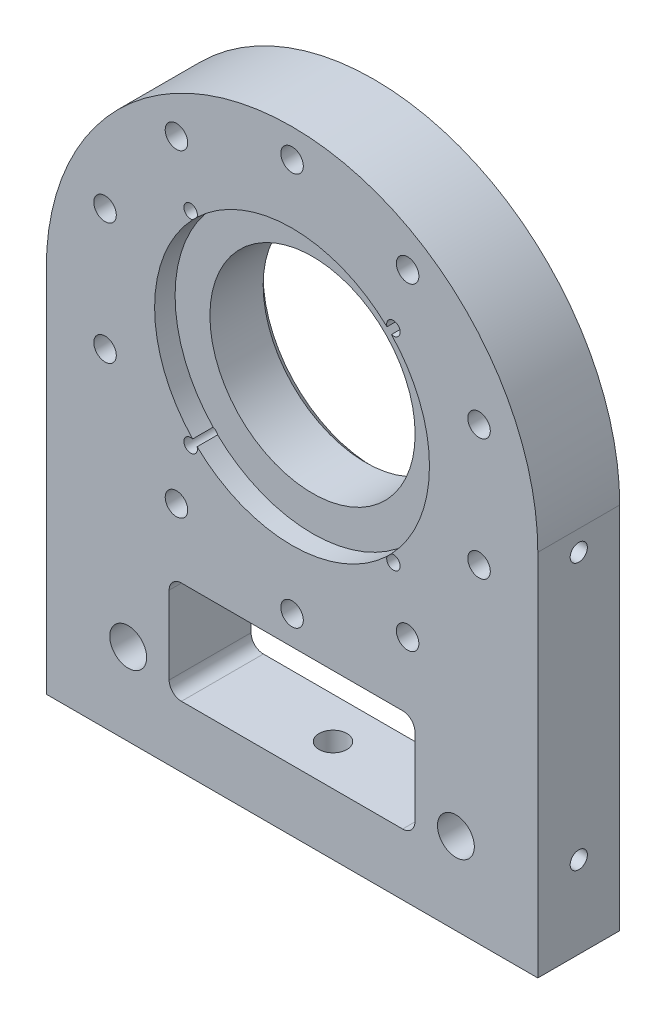
from build123d import *

# Parameters (mm, degrees)
SKETCH_1_R                  = 25.05
EXTRUDE_1_DEPTH             = 10
HOLE_WIZARD_M8_1_D          = 6.8
HOLE_WIZARD_M8_1_DEPTH      = 33.75
HOLE_WIZARD_M8_1_TIP        = 2.042926105
HOLE_WIZARD_6_0_6_1_D       = 6
HOLE_WIZARD_6_0_6_1_DEPTH   = 15
HOLE_WIZARD_6_0_6_1_TIP     = 1.802581857
SKETCH_6_R                  = 33.55
CUT_EXTRUDE_1_DEPTH         = 5
HOLE_WIZARD_M4_1_D          = 3.3
PATTERN_CIRCULAR_1_COUNT    = 4
CHAMFER_1_SIZE              = 2
HOLE_WIZARD_2_D             = 5.5
HOLE_WIZARD_2_CBORE_D       = 10
HOLE_WIZARD_2_CBORE_DEPTH   = 5.7
PATTERN_CIRCULAR_2_COUNT    = 10
HOLE_WIZARD_2_2_D           = 9
HOLE_WIZARD_2_2_CBORE_D     = 15
HOLE_WIZARD_2_2_CBORE_DEPTH = 9
CUT_EXTRUDE_2_DEPTH         = 163.788205961
HOLE_WIZARD_M5_1_AT_2_COUNT = 2
HOLE_WIZARD_M5_1_AT_2_PITCH = 65


with BuildPart() as part:
    # 草图1 → 凸台-拉伸1 (new, symmetric)
    with BuildSketch(Plane.XY):
        with BuildLine():
            Line((-60, 90), (-60, 0))
            Line((-60, 0), (60, 0))
            Line((60, 0), (60, 90))
            ThreePointArc((60, 90), (0, 150), (-60, 90))
        make_face()
        with Locations((0, 95)):
            Circle(SKETCH_1_R, mode=Mode.SUBTRACT)
    extrude(amount=EXTRUDE_1_DEPTH, both=True)

    # M8 螺纹孔1
    with Locations(Plane(origin=(0, 0, 0), x_dir=(-1, 0, 0), z_dir=(0, -1, 0))):
        with Locations((50, 0), (0, 0), (-50, 0)):
            Hole(HOLE_WIZARD_M8_1_D / 2, depth=HOLE_WIZARD_M8_1_DEPTH)
            with Locations((0, 0, -(HOLE_WIZARD_M8_1_DEPTH + HOLE_WIZARD_M8_1_TIP / 2))):  # 118° drill point
                Cone(0, HOLE_WIZARD_M8_1_D / 2, HOLE_WIZARD_M8_1_TIP, mode=Mode.SUBTRACT)

    # Ø6.0 (6) 直径孔1
    with Locations(Plane(origin=(0, 0, 0), x_dir=(-1, 0, 0), z_dir=(0, -1, 0))):
        with Locations((-35, 0), (35, 0)):
            Hole(HOLE_WIZARD_6_0_6_1_D / 2, depth=HOLE_WIZARD_6_0_6_1_DEPTH)
            with Locations((0, 0, -(HOLE_WIZARD_6_0_6_1_DEPTH + HOLE_WIZARD_6_0_6_1_TIP / 2))):  # 118° drill point
                Cone(0, HOLE_WIZARD_6_0_6_1_D / 2, HOLE_WIZARD_6_0_6_1_TIP, mode=Mode.SUBTRACT)

    # 草图6 → 切除-拉伸1 (cut)
    with BuildSketch(Plane.XY.offset(10)):
        with Locations((0, 95)):
            Circle(SKETCH_6_R)
    extrude(amount=-CUT_EXTRUDE_1_DEPTH, mode=Mode.SUBTRACT)

    # M4 螺纹孔1 (through all)
    with Locations(Plane(origin=(0, 0, -10), x_dir=(-1, 0, 0), z_dir=(0, 0, -1))):
        with Locations((-24.748737342, 119.748737342)):
            hole_wizard_m4_1 = Hole(HOLE_WIZARD_M4_1_D / 2)

    # 阵列(圆周)1: M4 螺纹孔1 ×4 about axis
    pattern_circular_1_axis = Axis((0, 95, 0), (0, 0, 1))
    for i in range(1, PATTERN_CIRCULAR_1_COUNT):
        add(hole_wizard_m4_1.rotate(pattern_circular_1_axis, i * 360 / PATTERN_CIRCULAR_1_COUNT), mode=Mode.SUBTRACT)

    # 倒角1
    chamfer_1_edges = [part.edges().sort_by_distance(p)[0] for p in [
        (-25.05, 95, -10),
    ]]
    chamfer(chamfer_1_edges, length=CHAMFER_1_SIZE)

    # Hole Wizard 2 (through all)
    with Locations(Plane(origin=(0, 0, -10), x_dir=(-1, 0, 0), z_dir=(0, 0, -1))):
        with Locations((0, 143)):
            hole_wizard_2 = CounterBoreHole(HOLE_WIZARD_2_D / 2, HOLE_WIZARD_2_CBORE_D / 2, HOLE_WIZARD_2_CBORE_DEPTH)

    # 阵列(圆周)2: Hole Wizard 2 ×10 about axis
    pattern_circular_2_axis = Axis((0, 95, 0), (0, 0, 1))
    for i in range(1, PATTERN_CIRCULAR_2_COUNT):
        add(hole_wizard_2.rotate(pattern_circular_2_axis, i * 360 / PATTERN_CIRCULAR_2_COUNT), mode=Mode.SUBTRACT)

    # Hole Wizard 2 2 (through all)
    with Locations(Plane(origin=(0, 0, -10), x_dir=(-1, 0, 0), z_dir=(0, 0, -1))):
        with Locations((-40, 20), (40, 20)):
            CounterBoreHole(HOLE_WIZARD_2_2_D / 2, HOLE_WIZARD_2_2_CBORE_D / 2, HOLE_WIZARD_2_2_CBORE_DEPTH)

    # 草图13 → 切除-拉伸2 (cut, through all)
    with BuildSketch(Plane(origin=(0, 0, -10), x_dir=(-1, 0, 0), z_dir=(0, 0, -1))):
        with BuildLine():
            Line((-27, 40), (27, 40))
            ThreePointArc((27, 40), (29.121320344, 39.121320344), (30, 37))
            Line((30, 37), (30, 18))
            ThreePointArc((30, 18), (29.121320344, 15.878679656), (27, 15))
            Line((27, 15), (-27, 15))
            ThreePointArc((-27, 15), (-29.121320344, 15.878679656), (-30, 18))
            Line((-30, 18), (-30, 37))
            ThreePointArc((-30, 37), (-29.121320344, 39.121320344), (-27, 40))
        make_face()
    extrude(amount=-CUT_EXTRUDE_2_DEPTH, mode=Mode.SUBTRACT)

    # 草图15 → M5 螺纹孔1 (revolve, cut)
    with BuildSketch(Plane(origin=(60, 20, 0), x_dir=(0, 0, -1), z_dir=(0, 1, 0))):
        Polygon((0, 0), (0, 15.6618073), (2.1, 14.4), (2.1, 0), align=None)
    hole_wizard_m5_1 = revolve(axis=Axis((66.35, 20, 0), (-1, 0, 0)), mode=Mode.SUBTRACT)

    # M5 螺纹孔1 at 2: M5 螺纹孔1 ×2
    with Locations(*[(0, i * HOLE_WIZARD_M5_1_AT_2_PITCH, 0) for i in range(1, HOLE_WIZARD_M5_1_AT_2_COUNT)]):
        add(hole_wizard_m5_1, mode=Mode.SUBTRACT)

    # 镜向1: M5 螺纹孔1 across plane
    add(hole_wizard_m5_1.mirror(Plane(origin=(0, 0, 0), x_dir=(0, 0, 1), z_dir=(1, 0, 0))), mode=Mode.SUBTRACT)

    # 镜向1 copy 1 sketch → 镜向1 copy 1 (revolve, cut)
    with BuildSketch(Plane(origin=(-60, 85, 0), x_dir=(0, 0, -1), z_dir=(0, 1, 0))):
        Polygon((0, 0), (0, -15.6618073), (2.1, -14.4), (2.1, 0), align=None)
    revolve(axis=Axis((-66.35, 85, 0), (-1, 0, 0)), mode=Mode.SUBTRACT)


solid = part.part
